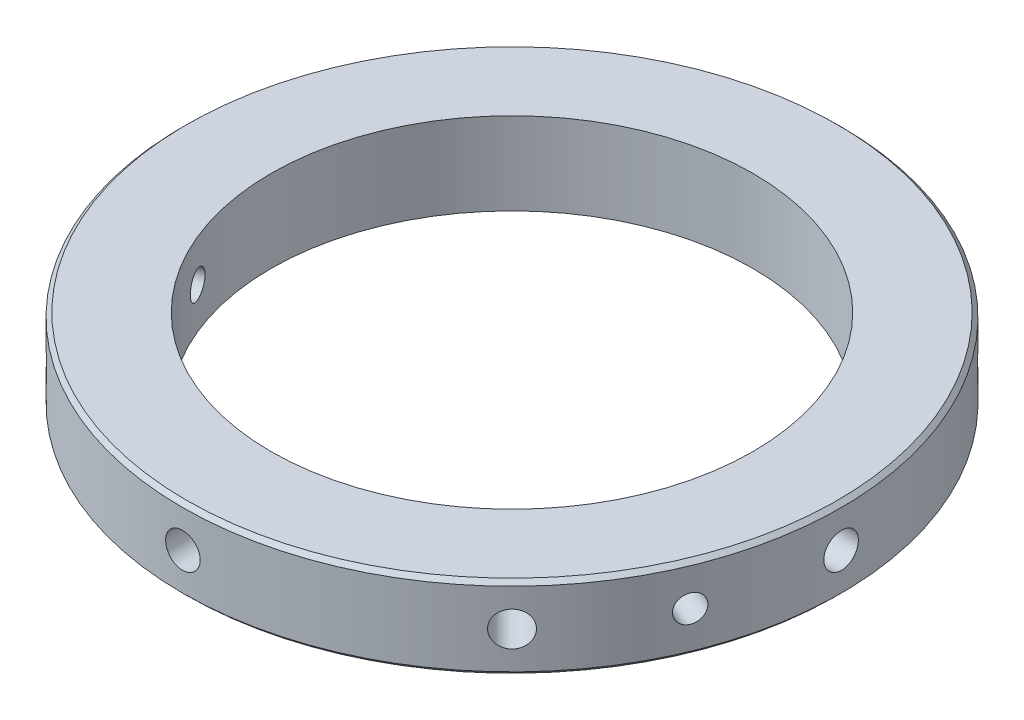
from build123d import *

# Parameters (mm, degrees)
SKETCH1_R              = 40
SKETCH1_R_2            = 29.25
BOSS_EXTRUDE1_DEPTH    = 5
CIRPATTERN1_COUNT      = 8
M4_TAPPED_HOLE1_REACH  = 96.9
M4_TAPPED_HOLE1_BORE_R = 1.65
CIRPATTERN2_COUNT      = 2
CIRPATTERN2_ANGLE      = 135
CHAMFER1_SIZE          = 0.5


with BuildPart() as part:
    # Sketch1 → Boss-Extrude1 (new, symmetric)
    with BuildSketch(Plane(origin=(0, 0, 0), x_dir=(1, 0, 0), z_dir=(0, 1, 0))):
        with Locations(Location((0, 0, 0), (0, 0, 270))):
            Circle(SKETCH1_R)
        with Locations(Location((0, 0, 0), (0, 0, 270))):
            Circle(SKETCH1_R_2, mode=Mode.SUBTRACT)
    extrude(amount=BOSS_EXTRUDE1_DEPTH, both=True)

    # Sketch2 → Ø4.2 (4.2) Diameter Hole1 (revolve, cut)
    with BuildSketch(Plane(origin=(0, 0, 40), x_dir=(0, -1, 0), z_dir=(1, 0, 0))):
        Polygon((0, 0), (0, 8.2618073), (2.1, 7), (2.1, 0), align=None)
    f_4_2_4_2_diameter_hole1 = revolve(axis=Axis((0, 0, 46.35), (0, 0, -1)), mode=Mode.SUBTRACT)

    # CirPattern1: Ø4.2 (4.2) Diameter Hole1 ×8 about axis
    cirpattern1_axis = Axis((0, 5, 0), (0, -1, 0))
    for i in range(1, CIRPATTERN1_COUNT):
        add(f_4_2_4_2_diameter_hole1.rotate(cirpattern1_axis, i * 360 / CIRPATTERN1_COUNT), mode=Mode.SUBTRACT)

    # M4 Tapped Hole1 bore → M4 Tapped Hole1 (cut, up to next)
    with BuildSketch(Plane(origin=(36.9551813, 0, 15.307337295), x_dir=(0.3826834323650906, 0, -0.9238795325112865), z_dir=(0.9238795325112864, 0, 0.38268343236509056)), mode=Mode.PRIVATE) as m4_tapped_hole1_sk1:
        Circle(M4_TAPPED_HOLE1_BORE_R)
    m4_tapped_hole1_tool1 = extrude(m4_tapped_hole1_sk1.sketch, amount=-M4_TAPPED_HOLE1_REACH, mode=Mode.PRIVATE) & part.part
    m4_tapped_hole1 = m4_tapped_hole1_tool1.solids().sort_by_distance((36.955181, 0, 15.307337))[0]
    add(m4_tapped_hole1, mode=Mode.SUBTRACT)

    # CirPattern2: M4 Tapped Hole1 ×2 about axis
    cirpattern2_axis = Axis((0, 5, 0), (0, -1, 0))
    for i in range(1, CIRPATTERN2_COUNT):
        add(m4_tapped_hole1.rotate(cirpattern2_axis, i * CIRPATTERN2_ANGLE / (CIRPATTERN2_COUNT - 1)), mode=Mode.SUBTRACT)

    # Chamfer1
    chamfer1_edges = [part.edges().sort_by_distance(p)[0] for p in [
        (0, -5, -40),
        (0, 5, -40),
    ]]
    chamfer(chamfer1_edges, length=CHAMFER1_SIZE)


solid = part.part
